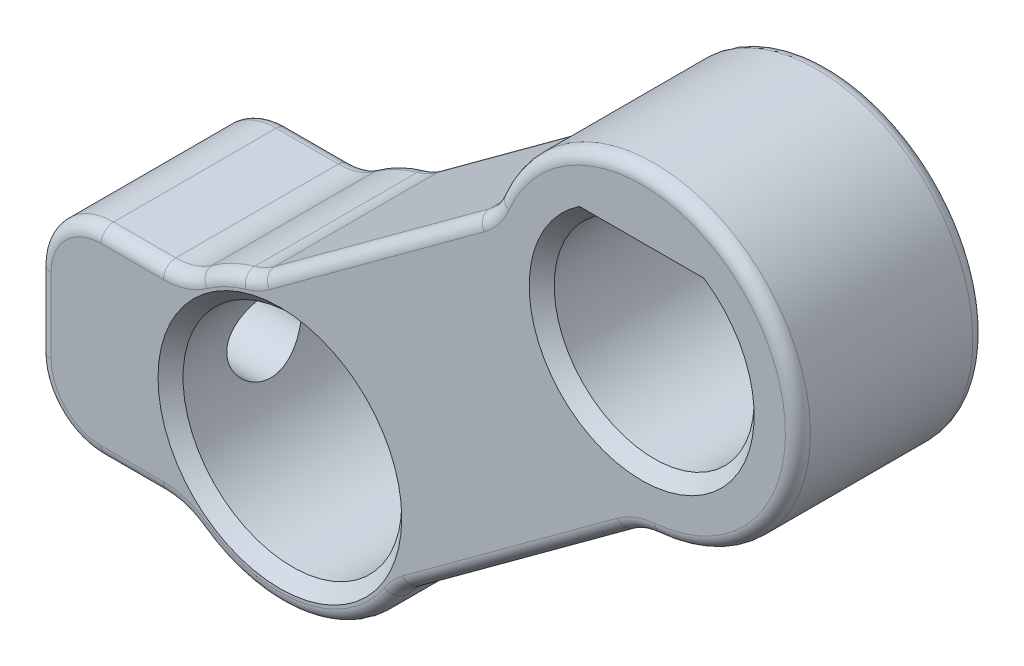
from build123d import *

# Parameters (mm, degrees)
SKETCH_1_R          = 17.5
EXTRUDE_1_DEPTH     = 30
FILLET_1_R          = 10
FILLET_2_R          = 2
CHAMFER_1_SIZE      = 2
SKETCH_2_R          = 6
CUT_EXTRUDE_1_DEPTH = 50


with BuildPart() as part:
    # 草图1 → 凸台-拉伸1 (new body)
    with BuildSketch(Plane.XY):
        with BuildLine():
            Line((-309.587406351, -15.805528725), (-347.990135407, -43.951995119))
            ThreePointArc((-347.990135407, -43.951995119), (-353.711105355, -45.983464105), (-358.659024526, -49.501199067))
            Line((-358.659024526, -49.501199067), (-382.159355655, -49.501199067))
            Line((-382.159355655, -49.501199067), (-382.159355655, -65.501199067))
            Line((-382.159355655, -65.501199067), (-382.159355655, -81.501199067))
            Line((-382.159355655, -81.501199067), (-358.659024526, -81.501199067))
            ThreePointArc((-358.659024526, -81.501199067), (-340.209418876, -87.244656096), (-324.344076601, -76.214417578))
            Line((-324.344076601, -76.214417578), (-285.941347545, -48.067951184))
            ThreePointArc((-285.941347545, -48.067951184), (-265.501954489, -8.290681148), (-309.587406351, -15.805528725))
        make_face()
        with Locations((-343.559355655, -65.501199067)):
            Circle(SKETCH_1_R, mode=Mode.SUBTRACT)
        with BuildLine():
            Line((-294.993347579, -10.069467902), (-276.338589473, -10.069467902))
            ThreePointArc((-276.338589473, -10.069467902), (-285.665968526, -39.069467902), (-294.993347579, -10.069467902))
        make_face(mode=Mode.SUBTRACT)
    extrude(amount=EXTRUDE_1_DEPTH)

    # 圆角1
    fillet_1_edges = [part.edges().sort_by_distance(p)[0] for p in [
        (-347.990135407, -43.951995119, 15),
        (-309.587406351, -15.805528725, 15),
        (-285.941347545, -48.067951184, 15),
        (-324.344076601, -76.214417578, 15),
        (-358.659024526, -81.501199067, 15),
        (-382.159355655, -81.501199067, 15),
        (-382.159355655, -49.501199067, 15),
        (-358.659024526, -49.501199067, 15),
    ]]
    fillet(fillet_1_edges, radius=FILLET_1_R)

    # 圆角2
    fillet_2_edges = [part.edges().sort_by_distance(p)[0] for p in [
        (-353.122981052, -45.688650789, 0),
        (-353.122981052, -45.688650789, 30),
        (-329.215190996, -30.191297509, 0),
        (-329.215190996, -30.191297509, 30),
        (-265.501954489, -8.290681148, 0),
        (-265.501954489, -8.290681148, 30),
        (-305.56913219, -62.453719969, 0),
        (-305.56913219, -62.453719969, 30),
        (-339.560781684, -87.134770344, 0),
        (-339.560781684, -87.134770344, 30),
        (-367.186734708, -81.501199067, 0),
        (-367.186734708, -81.501199067, 30),
        (-382.159355655, -65.501199067, 0),
        (-367.186734708, -49.501199067, 0),
        (-379.230423467, -52.430131255, 0),
        (-379.230423467, -78.572266879, 0),
        (-382.159355655, -65.501199067, 30),
        (-367.186734708, -49.501199067, 30),
        (-379.230423467, -52.430131255, 30),
        (-379.230423467, -78.572266879, 30),
        (-347.919818401, -43.705196344, 0),
        (-347.919818401, -43.705196344, 30),
        (-310.08888806, -15.722079028, 0),
        (-310.08888806, -15.722079028, 30),
        (-324.087558519, -76.221669503, 0),
        (-324.087558519, -76.221669503, 30),
        (-359.152251583, -81.981482685, 0),
        (-359.152251583, -81.981482685, 30),
        (-359.152251583, -49.020915449, 0),
        (-359.152251583, -49.020915449, 30),
        (-286.012756057, -48.571288626, 0),
        (-286.012756057, -48.571288626, 30),
    ]]
    fillet(fillet_2_edges, radius=FILLET_2_R)

    # 倒角1
    chamfer_1_edges = [part.edges().sort_by_distance(p)[0] for p in [
        (-285.665968526, -39.069467902, 0),
        (-285.665968526, -10.069467902, 0),
        (-285.665968526, -39.069467902, 30),
        (-285.665968526, -10.069467902, 30),
        (-361.059355655, -65.501199067, 0),
        (-361.059355655, -65.501199067, 30),
    ]]
    chamfer(chamfer_1_edges, length=CHAMFER_1_SIZE)

    # 草图2 → 切除-拉伸1 (cut)
    with BuildSketch(Plane.ZY.offset(382.159355655)):
        with Locations((15, -65.501199067)):
            Circle(SKETCH_2_R)
    extrude(amount=-CUT_EXTRUDE_1_DEPTH, mode=Mode.SUBTRACT)


solid = part.part
